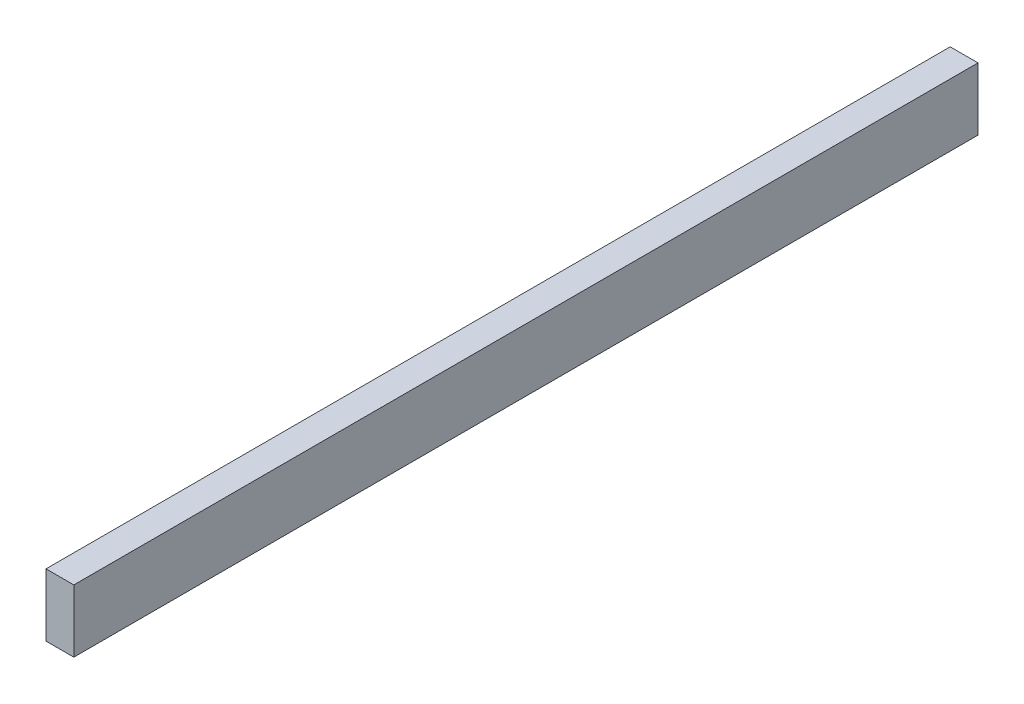
from build123d import *

# Parameters (mm, degrees)
SKETCH_1_W      = 8
SKETCH_1_H      = 18
EXTRUDE_1_DEPTH = 130


with BuildPart() as part:
    # 草图1 → 凸台-拉伸1 (new, symmetric)
    with BuildSketch(Plane.XY):
        Rectangle(SKETCH_1_W, SKETCH_1_H)
    extrude(amount=EXTRUDE_1_DEPTH, both=True)


solid = part.part
